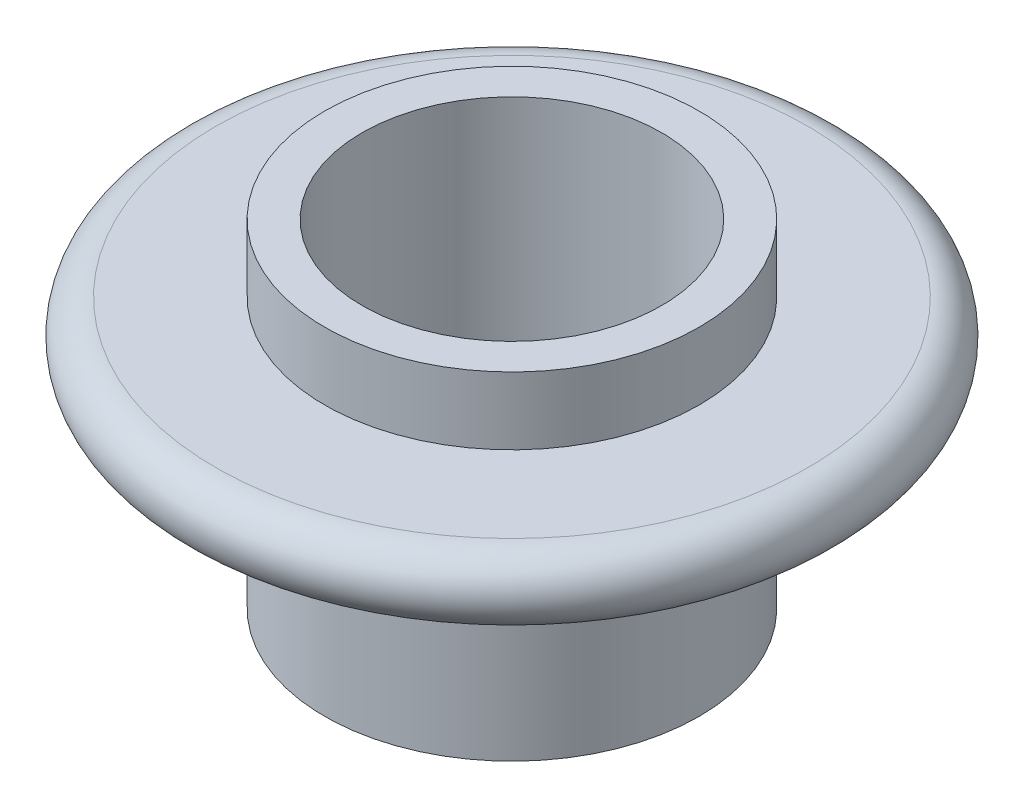
SolidWorks part; units mm, degrees
ref_plane "Front Plane" through (0, 0, 0) normal (0, 0, 1) x (1, 0, 0)
ref_plane "Top Plane" through (0, 0, 0) normal (0, 1, 0) x (1, 0, 0)
ref_plane "Right Plane" through (0, 0, 0) normal (1, 0, 0) x (0, 0, -1)
sketch "Sketch1" plane through (0, 0, 0) normal (0, 0, 1) x (1, 0, 0)
  line L0 (0, 22.5) -> (0, -22.5) construction
  line L1 (20, 22.5) -> (20, -22.5)
  line L2 (20, -22.5) -> (25, -22.5)
  line L3 (25, -22.5) -> (25, 4.5)
  line L4 (25, 4.5) -> (39.5, 4.5)
  line L6 (39.5, 13.5) -> (25, 13.5)
  line L7 (25, 13.5) -> (25, 22.5)
  line L8 (25, 22.5) -> (20, 22.5)
  line L9 (44, 9) -> (39.5, 9) construction
  arc A0 (39.5, 4.5) -> (39.5, 13.5) centre (39.5, 9) ccw
  dimension "D1" = 45
  dimension "D2" = 9
  dimension "D4" = 27
  dimension "D6" = 40
  dimension "D7" = 50
  dimension "D8" = 50
  dimension "D9" = 4.5
revolve "Revolve1" add sketch "Sketch1" angle 360 about L0
